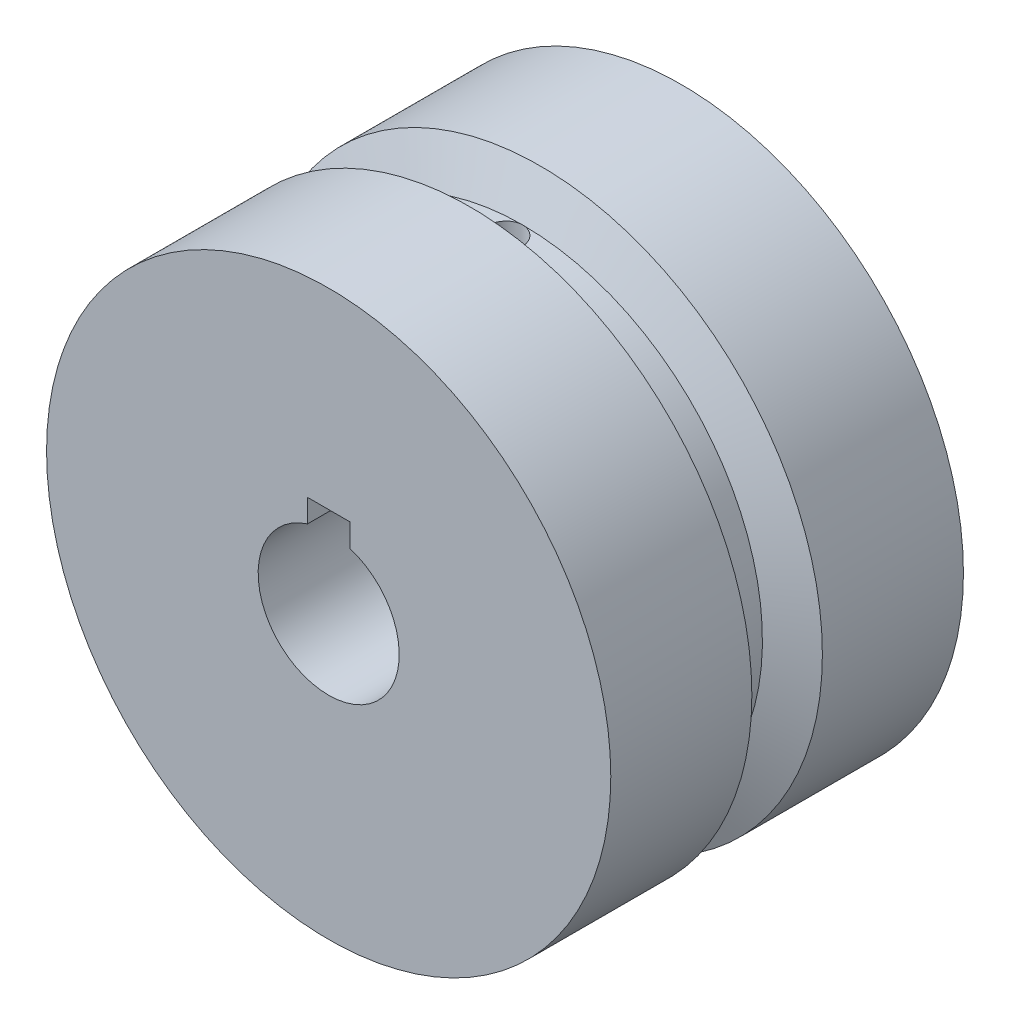
from build123d import *
from build123d.topology import SkipClean

# Parameters (mm, degrees)
SKETCH_1_R               = 40
SKETCH_1_R_2             = 10
EXTRUDE_1_DEPTH          = 25
SKETCH_6_W               = 6
SKETCH_6_H               = 9.759677648
CUT_EXTRUDE_1_DEPTH      = 76.498344353
SKETCH_8_W               = 2.1
SKETCH_8_H               = 40
CUT_EXTRUDE_START        = 40
SKETCH_9_R               = 2.5
CUT_EXTRUDE_2_DEPTH      = 20
PATTERN_CIRCULAR_1_COUNT = 2
PATTERN_CIRCULAR_1_ANGLE = 90


with BuildPart() as part:
    # 草图1 → 凸台-拉伸1 (new, symmetric)
    with BuildSketch(Plane.XY):
        Circle(SKETCH_1_R)
        Circle(SKETCH_1_R_2, mode=Mode.SUBTRACT)
    extrude(amount=EXTRUDE_1_DEPTH, both=True)

    # 草图5 → 切除-旋转1 (revolve, cut)
    with BuildSketch(Plane(origin=(0, 0, 0), x_dir=(1, 0, 0), z_dir=(0, 1, 0)), mode=Mode.PRIVATE) as cut_revolve_1_sk:
        Polygon((-40, -5), (-40, 5), (-34, 2.5), (-34, -2.5), align=None)
    revolve(cut_revolve_1_sk.sketch.rotate(Axis((0, 0, 0), (0, 0, -1)), 180), axis=Axis((0, 0, 0), (0, 0, -1)), mode=Mode.SUBTRACT)

    # 草图6 → 切除-拉伸1 (cut, through all)
    with BuildSketch(Plane.XY.offset(25)):
        with Locations((0, 7.920161176)):
            Rectangle(SKETCH_6_W, SKETCH_6_H)
    extrude(amount=-CUT_EXTRUDE_1_DEPTH, mode=Mode.SUBTRACT)

    # 草图8 → M5 螺纹孔1 (revolve, cut)
    with BuildSketch(Plane(origin=(0, 0, 0), x_dir=(0, 0, -1), z_dir=(1, 0, 0))):
        with Locations((1.05, 20)):
            Rectangle(SKETCH_8_W, SKETCH_8_H)
    hole_wizard_m5_1 = revolve(axis=Axis((0, -6.35, 0), (0, 1, 0)), mode=Mode.SUBTRACT)

    # 草图9 → 切除-拉伸2 (cut)
    with SkipClean():  # the faces are left unmerged after this step: merging them gives an invalid solid
        with BuildSketch(Plane(origin=(0, 0, 0), x_dir=(1, 0, 0), z_dir=(0, 1, 0)).offset(CUT_EXTRUDE_START)):
            with Locations(Location((0, 0, 0), (0, 0, 270))):
                Circle(SKETCH_9_R)
        cut_extrude_2 = extrude(amount=-CUT_EXTRUDE_2_DEPTH, mode=Mode.SUBTRACT)

    # 阵列(圆周)1: M5 螺纹孔1, 切除-拉伸2 ×2 about axis
    pattern_circular_1_axis = Axis((0, 0, 25), (0, 0, 1))
    add([hole_wizard_m5_1.rotate(pattern_circular_1_axis, i * PATTERN_CIRCULAR_1_ANGLE / (PATTERN_CIRCULAR_1_COUNT - 1)) for i in range(1, PATTERN_CIRCULAR_1_COUNT)], mode=Mode.SUBTRACT)
    add([cut_extrude_2.rotate(pattern_circular_1_axis, i * PATTERN_CIRCULAR_1_ANGLE / (PATTERN_CIRCULAR_1_COUNT - 1)) for i in range(1, PATTERN_CIRCULAR_1_COUNT)], mode=Mode.SUBTRACT)


solid = part.part
